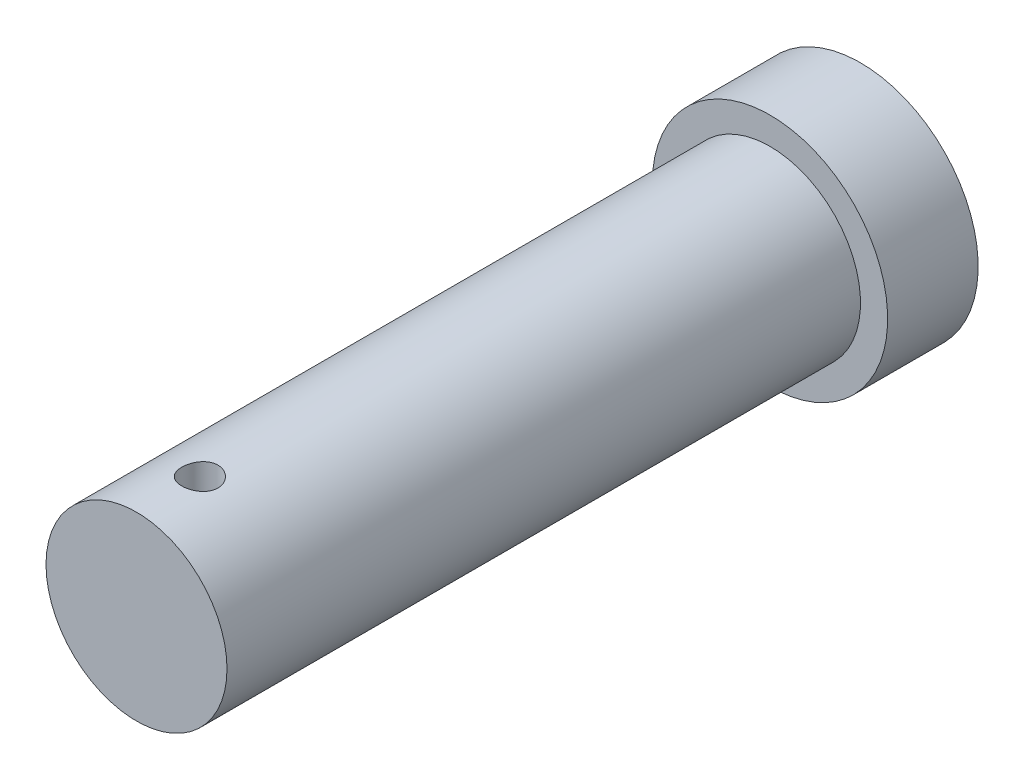
from build123d import *

# Parameters (mm, degrees)
SKETCH1_R               = 10
BOSS_EXTRUDE1_DEPTH     = 70
SKETCH2_R               = 13
BOSS_EXTRUDE2_DEPTH     = 10
CUT_EXTRUDE1_DEPTH      = 73.374028491
CUT_EXTRUDE1_DEPTH_BACK = 73.374028491
SKETCH3_R               = 2


with BuildPart() as part:
    # Sketch1 → Boss-Extrude1 (new body)
    with BuildSketch(Plane.XY):
        Circle(SKETCH1_R)
    extrude(amount=BOSS_EXTRUDE1_DEPTH)

    # Sketch2 → Boss-Extrude2 (add)
    with BuildSketch(Plane(origin=(0, 0, 0), x_dir=(-1, 0, 0), z_dir=(0, 0, -1))):
        Circle(SKETCH2_R)
    extrude(amount=BOSS_EXTRUDE2_DEPTH)

    # Sketch3 → Cut-Extrude1 (cut, two sides: drawn at the far end of the back side and taken through both)
    with BuildSketch(Plane(origin=(0, 0, 0), x_dir=(1, 0, 0), z_dir=(0, 1, 0)).offset(-CUT_EXTRUDE1_DEPTH_BACK)):
        with Locations(Location((0, -63, 0), (0, 0, 270))):
            Circle(SKETCH3_R)
    extrude(amount=CUT_EXTRUDE1_DEPTH + CUT_EXTRUDE1_DEPTH_BACK, mode=Mode.SUBTRACT)


solid = part.part
